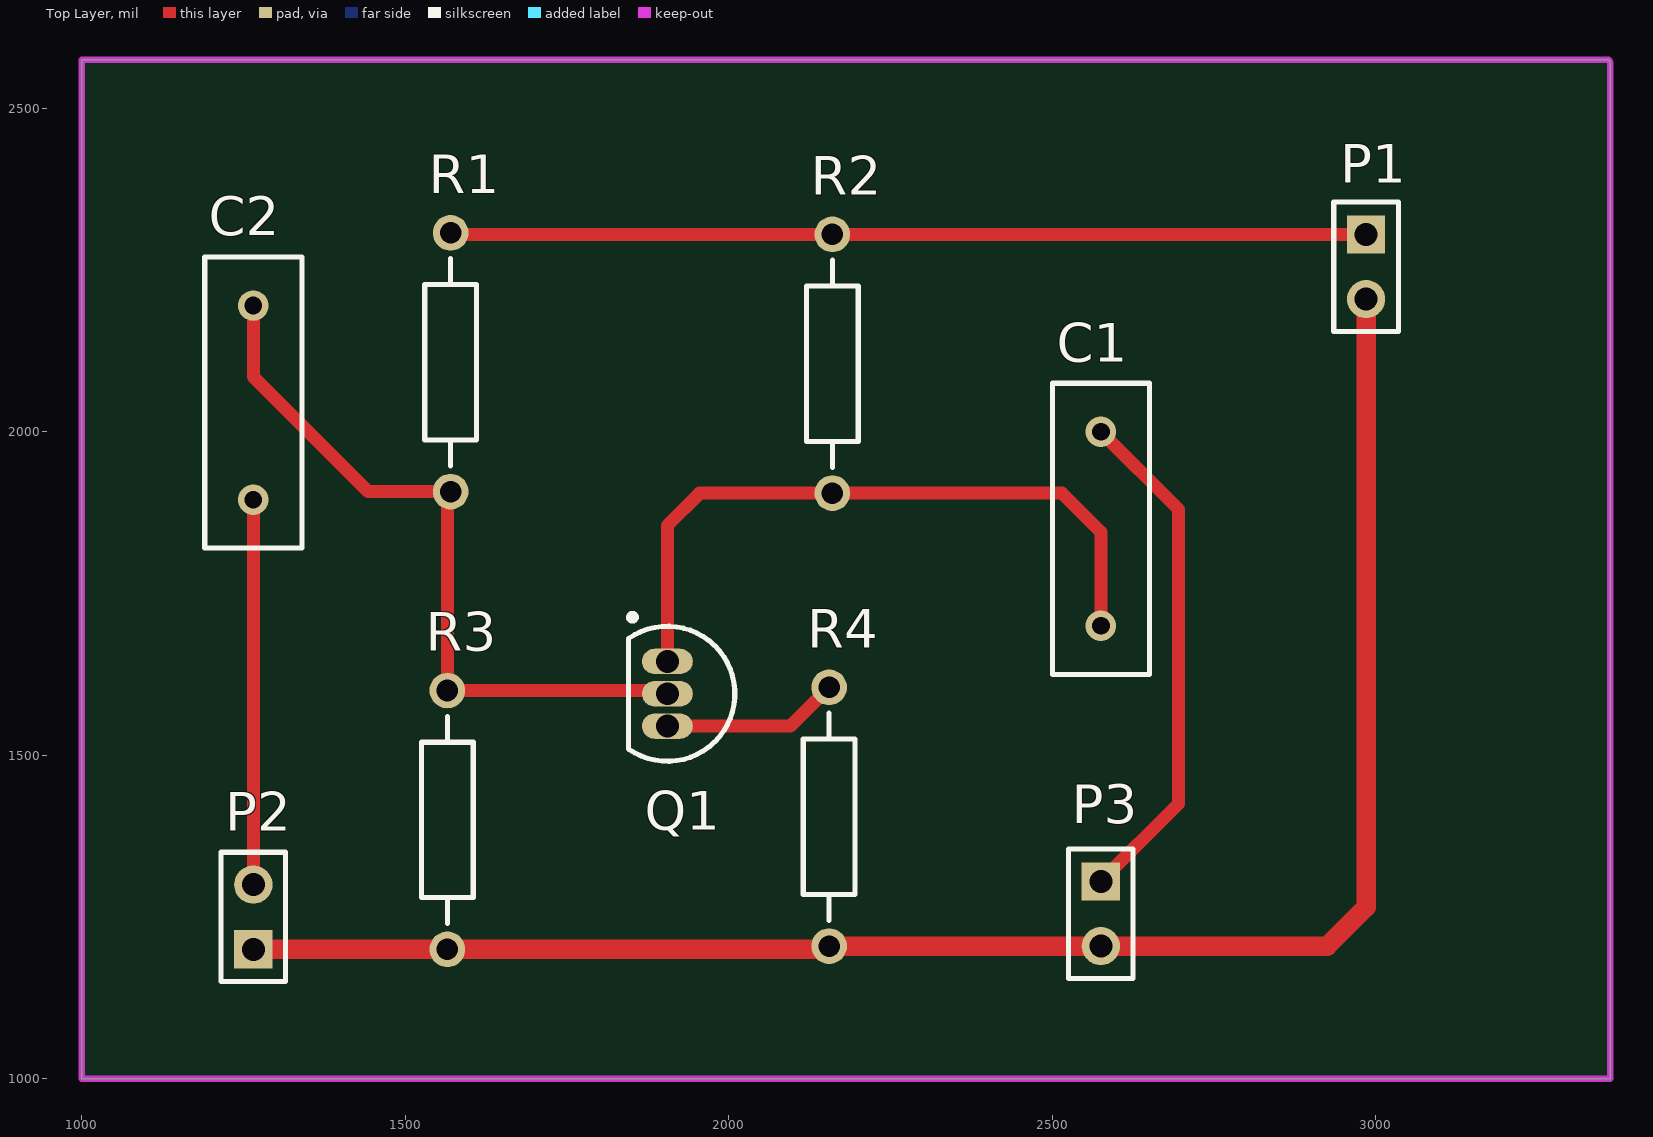
[diagram p0: Top Layer view]
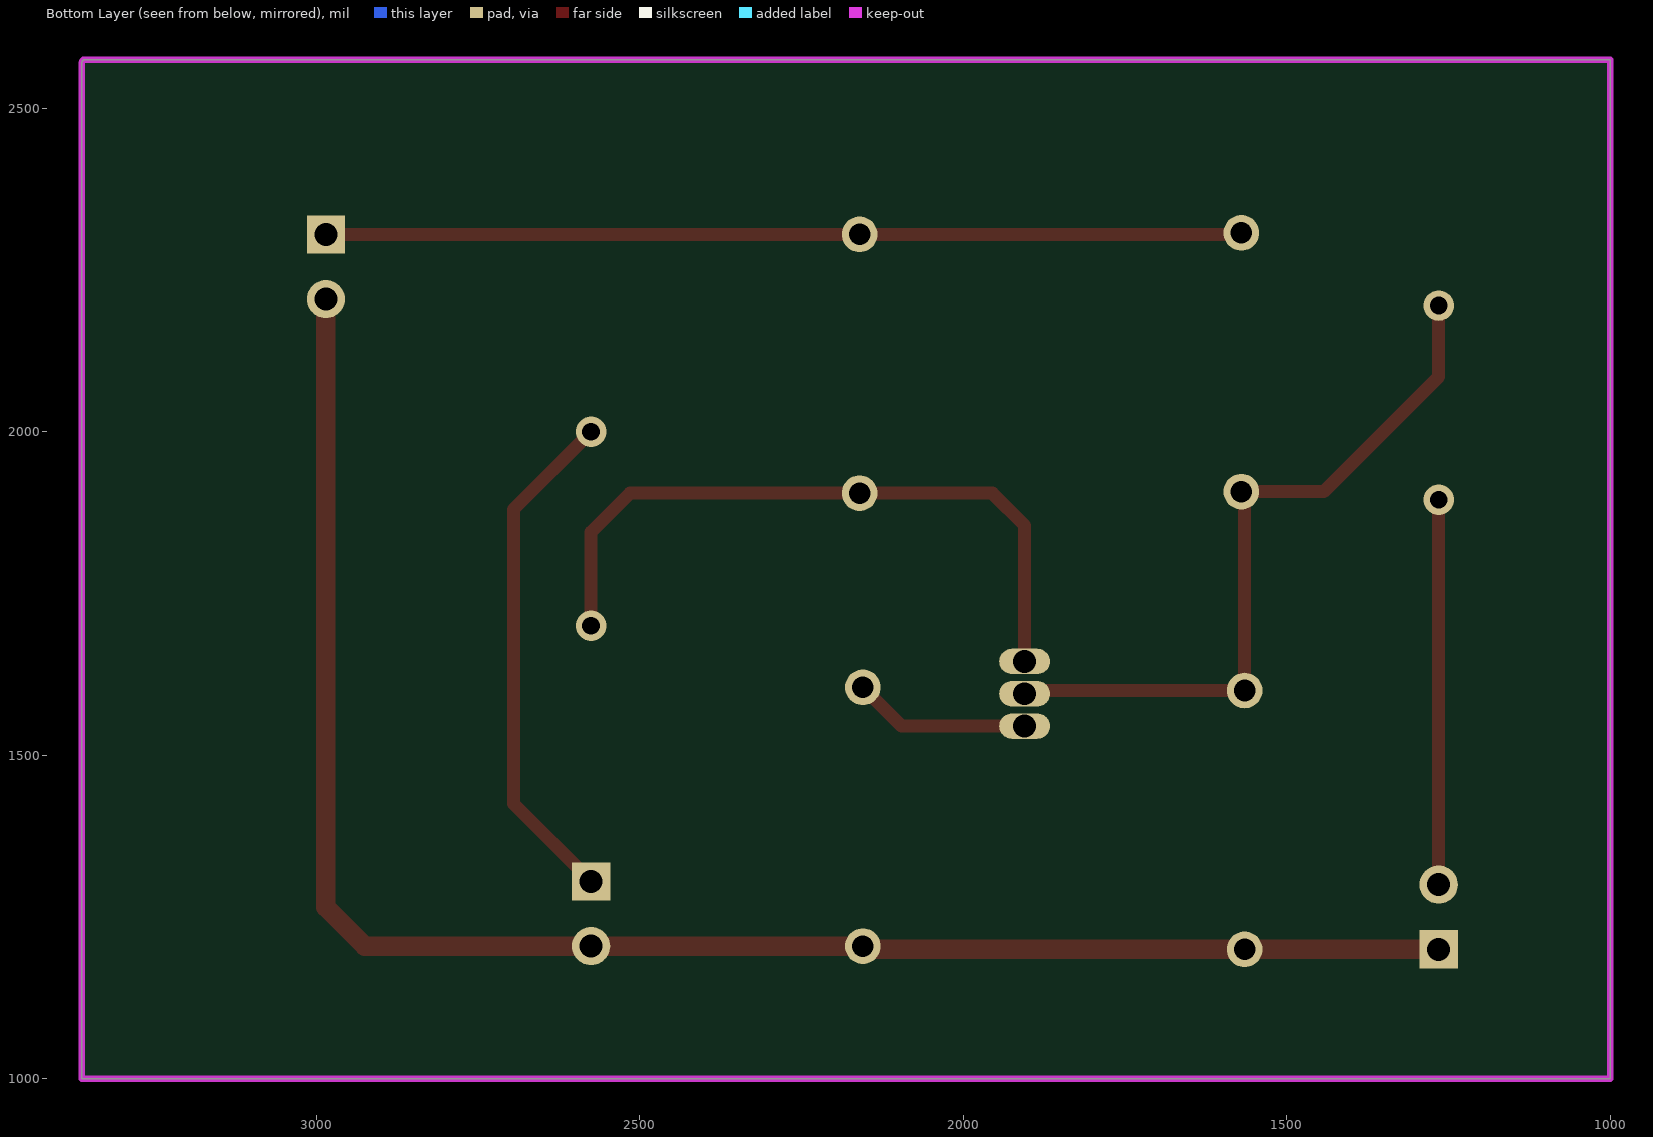
[diagram p1: Bottom Layer view, seen from below]
# Altium PCB MISC80548.PcbDoc
Units mil, origin at the board's own origin, x right, y up, seen from the top; angles counter-clockwise.
Board outline 2362.2 x 1574.8 mil, 2 copper layers (Top Layer, Bottom Layer); 10 components, 7 nets, 21 pads, 0 vias.

## Layer stack, top to bottom (the 12.6 mil dielectric is the usual default, probably not edited)
Top Solder: solder mask 0.4, Solder Resist, Dk 3.5
Top Layer: signal copper 1.4
Dielectric 1: dielectric 12.6, FR-4, Dk 4.8
Bottom Layer: signal copper 1.4
Bottom Solder: solder mask 0.4, Solder Resist, Dk 3.5

## Board outline
1000,1000 1000,2574.8 3360,2574.8 cw(c3354.68,2569.48) 3362.2,2569.48 3362.2,1000

## Design rules (kind name [scope] priority, off if disabled: settings)
Clearance [All] p1: gap=10
PolygonConnect [All] p1: connectstyle=Relief reliefconductorwidth=10 reliefentries=4 polygonreliefangle="90 Angle" airgapwidth=10
RoutingVias [All] p1: holewidth=28 width=50 viastyle="Through Hole" minholewidth=28 minwidth=50 maxholewidth=28 maxwidth=50
SolderMaskExpansion [All] p1: expansion=4
Width [All] p1: maxlimit=21850.39 minlimit=10 preferedwidth=10
30 further rules are at their usual default settings.

## Components (designator, comment, footprint, x,y, rotation, side; value= is the part's Value field where it differs from the comment)
C1 "100pF" RAD-0.3 2575,1850 r90 top
C2 "100pF" RAD-0.3 1265,2045 r90 top
P1 "Header 2" HDR1X2 2985,2305 r270 top
P2 "Header 2" HDR1X2 1265,1200 r90 top
P3 "Header 2" HDR1X2 2575,1305 r270 top
Q1 "NPN" TO-226-AA 1905,1595 r180 top
R1 "1K" AXIAL-0.4 1570,2107.38 r90 top
R2 "1K" AXIAL-0.4 2160,2105 r90 top
R3 "1K" AXIAL-0.4 1565,1400 r90 top
R4 "1K" AXIAL-0.4 2155,1405 r90 top

## Footprints (in the part's own frame and the unit in brackets; to place one, negate y for a bottom-side part, rotate by r counter-clockwise, add the part's x,y. Pads: shape width x height; smd on the part's side, far side on the other; paste and mask are expansions set on the pad)
AXIAL-0.4 [mm] "Axial Device, Thru-Hole; 2 Leads; 0.4 in Pin Spacing"
  round 1.4 hole 0.85: 1(-5.08,0) 2(5.08,0)
  silkscreen extent -4.06,-1.02 4.06,1.02
HDR1X2 [mm] "Connector; Header; 2 Position"
  rect 1.5x1.5 hole 0.9: 1(0,0)
  round 1.5 hole 0.9: 2(2.54,0)
  silkscreen extent -1.27,-1.27 3.81,1.27
RAD-0.3 [mm] "Radial Cap, Thru-Hole; 2 Leads; 0.3 in Pin Spacing"
  round 1.2 hole 0.7: 1(-3.81,0) 2(3.81,0)
  silkscreen extent -5.71,-1.91 5.71,1.91
TO-226-AA [mm] "TO, Flat Index; 3 In-Line, Axial Leads; Body Dia. 4.8mm; Leads 0.55 x 0.51 mm (max)"
  oval 2x1 hole 0.9: 1(0,-1.27) 2(0,0) 3(0,1.27)
  silkscreen extent -2.65,-3.13 1.52,2.65, body extent -2.65,-2.66 1.52,2.66, height 5.33

## Part data
C1 C2: library part Cap, "Capacitor"
P1 P2 P3: "Header, 2-Pin"
Q1: "NPN Bipolar Transistor"
R1 R2 R3 R4: library part Res2, "Resistor"

## Nets (pads, with @x,y where several pads share a name; then routed paths per layer and width w, separated by ;. In a path a pad name is that pad's centre, name@x,y a point inside that pad or via, vN(x,y) a via of type N, cw(c..) or ccw(c..) an arc to the next point about the centre after c; other vN are vias at no path point)
GND: P1.2 P2.1 P3.2 R3.1 R4.1 | length 2686.9
  Top Layer w30: P2.1 R3.1 2150,1200 R4.1 P3.2 2925,1205 2985,1265 P1.2
NetC1_1: C1.1 Q1.1 R2.1 | length 1070.6
  Top Layer w20: Q1.1 1905,1855 1955,1905 R2.1 2515,1905 2575,1845 C1.1
NetC1_2: C1.2 P3.1 | length 794.4
  Top Layer w20: P3.1 2695,1425 2695,1880 C1.2
NetC2_1: C2.1 P2.2 | length 595
  Top Layer w20: P2.2 C2.1
NetC2_2: C2.2 Q1.2 R1.1 R3.2 | length 1140.1
  Top Layer w20: C2.2 1265,2085 1442.62,1907.38 R1.1 1565,1902.38 R3.2 1900,1600 Q1.2
NetP1_1: P1.1 R1.2 R2.2 | length 1416
  Top Layer w20: R1.2 1572.38,2305 R2.2 P1.1
NetQ1_3: Q1.3 R4.2 | length 274.9
  Top Layer w20: Q1.3 2095,1545 R4.2

## Keep-outs
Keep-Out Layer:
  the board outline again, w10